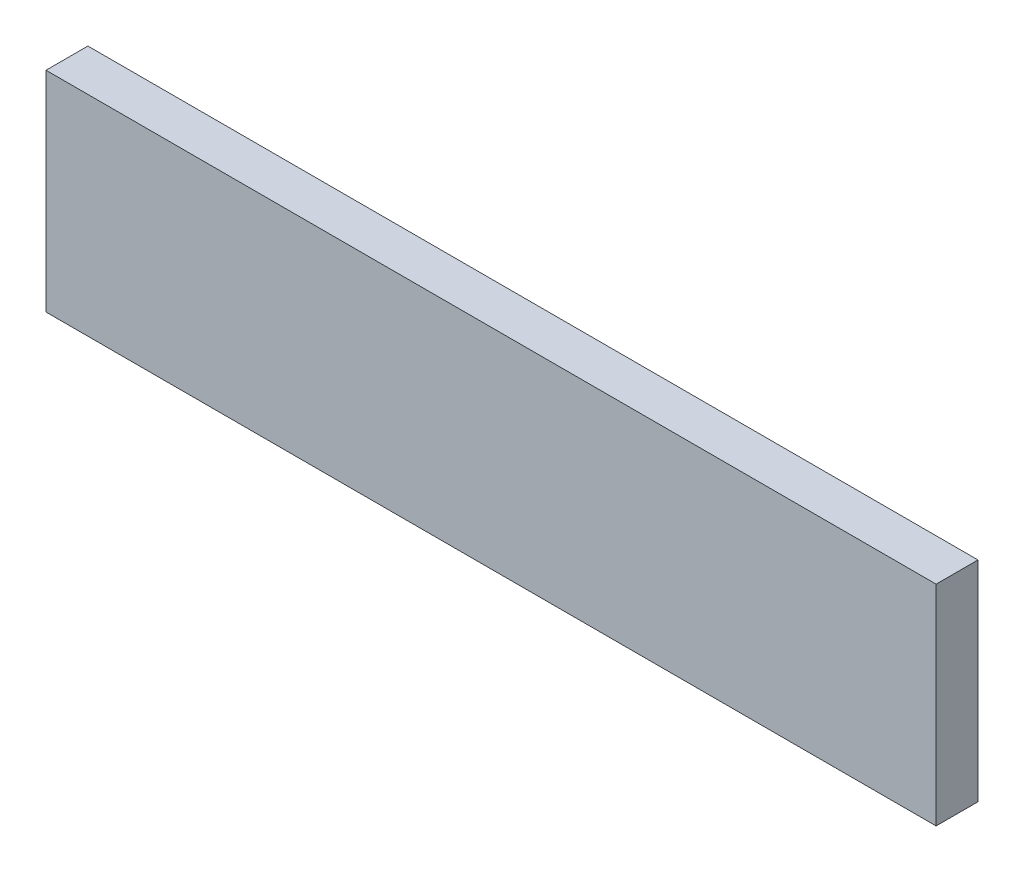
SolidWorks part; units mm, degrees
material "Q235"
ref_plane "Front Plane" through (0, 0, 0) normal (0, 0, 1) x (1, 0, 0)
ref_plane "Top Plane" through (0, 0, 0) normal (0, 1, 0) x (1, 0, 0)
ref_plane "Right Plane" through (0, 0, 0) normal (1, 0, 0) x (0, 0, -1)
sketch "Sketch1" plane through (0, 0, 0) normal (0, 0, 1) x (1, 0, 0)
  line L1 (0, 0) -> (425, 0)
  line L2 (0, 0) -> (0, 100)
  line L3 (0, 100) -> (425, 100)
  line L4 (425, 0) -> (425, 100)
  dimension "D1" = 425
  dimension "D2" = 100
extrude "Boss-Extrude1" add sketch "Sketch1" along normal blind 20
